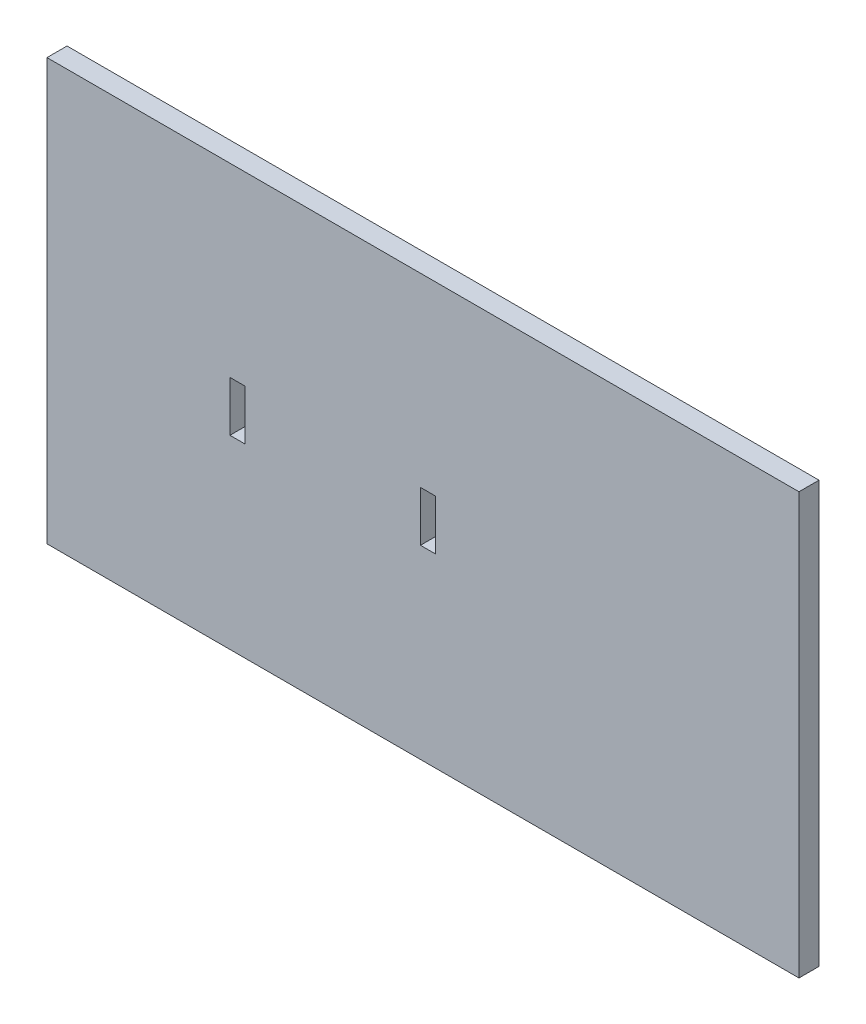
from build123d import *

# Parameters (mm, degrees)
SKETCH1_W           = 1500
SKETCH1_H           = 840
SKETCH1_W_2         = 30
SKETCH1_H_2         = 100
BOSS_EXTRUDE1_DEPTH = 40


with BuildPart() as part:
    # Sketch1 → Boss-Extrude1 (new body)
    with BuildSketch(Plane.XY):
        with Locations((750, 420)):
            Rectangle(SKETCH1_W, SKETCH1_H)
        with Locations((380, 420)):
            Rectangle(SKETCH1_W_2, SKETCH1_H_2, mode=Mode.SUBTRACT)
        with Locations((760, 420)):
            Rectangle(SKETCH1_W_2, SKETCH1_H_2, mode=Mode.SUBTRACT)
    extrude(amount=BOSS_EXTRUDE1_DEPTH)


solid = part.part
